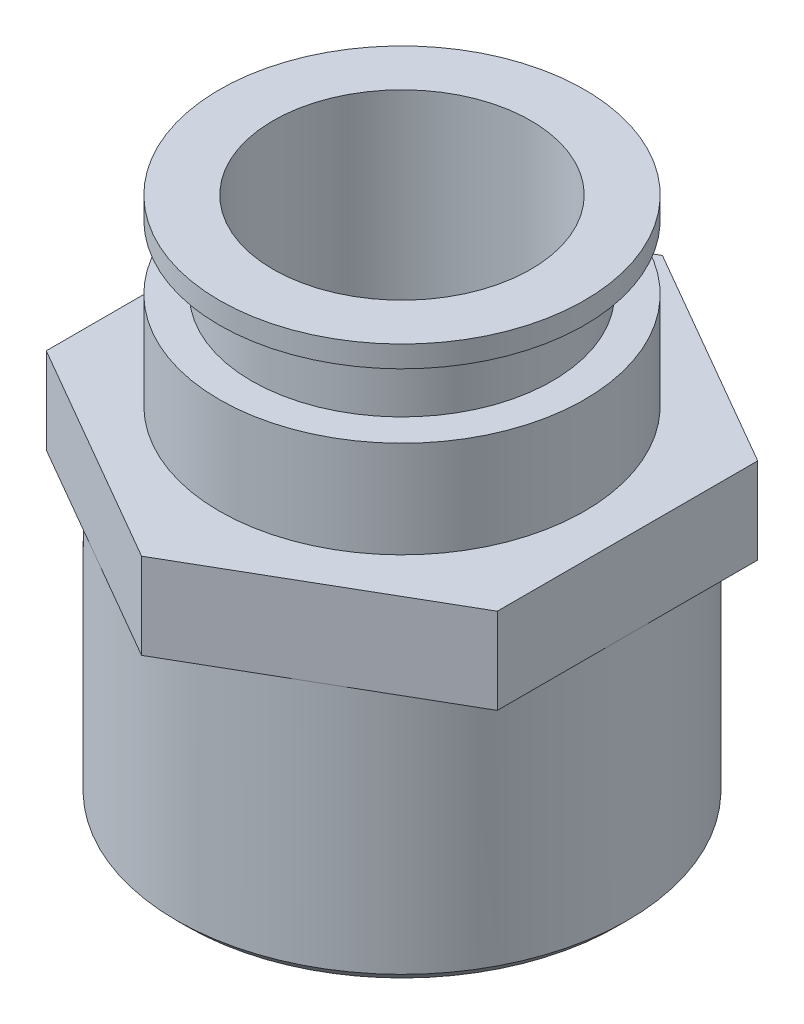
SolidWorks part; units mm, degrees
ref_plane "Front Plane" through (0, 0, 0) normal (0, 0, 1) x (1, 0, 0)
ref_plane "Top Plane" through (0, 0, 0) normal (0, 1, 0) x (1, 0, 0)
ref_plane "Right Plane" through (0, 0, 0) normal (1, 0, 0) x (0, 0, -1)
sketch "Sketch2" plane through (0, 0, 0) normal (0, 1, 0) x (1, 0, 0)
  circle A0 centre (0, 0) radius 10.5
  dimension "D1" = 21
extrude "Boss-Extrude1" add sketch "Sketch2" along normal blind 12
cosmetic thread "Cosmetic Thread2" parameters "D2"=18.632
sketch "Sketch3" plane through (0, 12, 0) normal (0, 1, 0) x (1, 0, 0)
  line L1 (10.5, -6.0622) -> (10.5, 6.0622)
  line L2 (10.5, 6.0622) -> (0, 12.1244)
  line L3 (0, 12.1244) -> (-10.5, 6.0622)
  line L4 (-10.5, 6.0622) -> (-10.5, -6.0622)
  line L5 (-10.5, -6.0622) -> (0, -12.1244)
  line L6 (0, -12.1244) -> (10.5, -6.0622)
  circle A0 centre (0, 0) radius 10.5 construction
  dimension "D1" = 21
extrude "Boss-Extrude2" add sketch "Sketch3" along normal blind 4
sketch "Sketch4" plane through (0, 16, 0) normal (0, 1, 0) x (1, 0, 0)
  circle A2 centre (0, 0) radius 8.5
  dimension "D1" = 17
extrude "Boss-Extrude3" add sketch "Sketch4" along normal blind 4.5
sketch "Sketch5" plane through (0, 20.5, 0) normal (0, 1, 0) x (1, 0, 0)
  circle A0 centre (0, 0) radius 7
  dimension "D1" = 14
extrude "Boss-Extrude4" add sketch "Sketch5" along normal blind 3
sketch "Sketch7" plane through (0, 23.5, 0) normal (0, 1, 0) x (1, 0, 0)
  circle A0 centre (0, 0) radius 8.5
  dimension "D1" = 17
extrude "Boss-Extrude5" add sketch "Sketch7" along normal blind 1
chamfer "Chamfer1" distance 0.5 angle 45 1 edges at (0, 0, 10.5)
sketch "Sketch8" plane through (0, 0, 0) normal (0, -1, 0) x (1, 0, 0)
  circle A0 centre (0, 0) radius 5
  dimension "D1" = 10
sketch "Sketch9" plane through (0, 24.5, 0) normal (0, 1, 0) x (1, 0, 0)
  circle A0 centre (0, 0) radius 6
  dimension "D1" = 12
extrude "Cut-Extrude1" cut sketch "Sketch9" against normal blind 11
extrude "Cut-Extrude2" cut sketch "Sketch8" against normal through all
